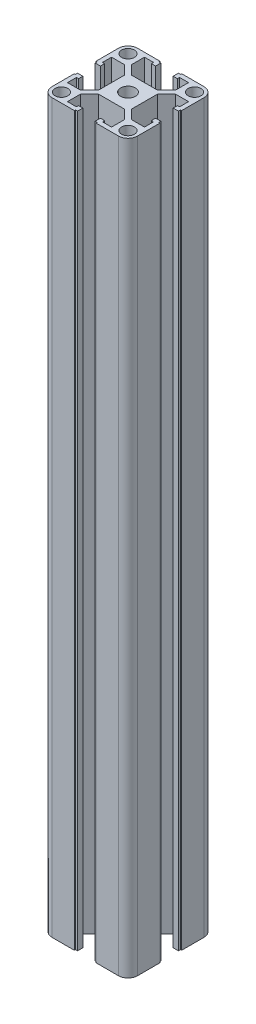
from build123d import *

# Parameters (mm, degrees)
SKETCH16_R             = 3.4
SKETCH16_R_2           = 3
MEMBER_1_DEPTH         = 340
HOLE_WIZARD_M8_3_D     = 6.9
HOLE_WIZARD_M8_3_DEPTH = 19.75
HOLE_WIZARD_M8_3_TIP   = 2.072969136


with BuildPart() as part:
    # Sketch16 → Member 1 (new body)
    with BuildSketch(Plane(origin=(0, 0, 0), x_dir=(-1, 0, 0), z_dir=(0, 1, 0))):
        with BuildLine():
            Line((-5.1, 20), (-5.1, 19.5))
            Line((-5.1, 19.5), (-4.1, 19.5))
            Line((-4.1, 19.5), (-4.1, 17))
            Line((-4.1, 17), (-6.1, 17))
            Line((-6.1, 17), (-6.1, 18))
            Line((-6.1, 18), (-10.3, 18))
            Line((-10.3, 18), (-10.3, 12))
            Line((-10.3, 12), (-6, 7.7))
            Line((-6, 7.7), (6, 7.7))
            Line((6, 7.7), (10.3, 12))
            Line((10.3, 12), (10.3, 18))
            Line((10.3, 18), (6.1, 18))
            Line((6.1, 18), (6.1, 17))
            Line((6.1, 17), (4.1, 17))
            Line((4.1, 17), (4.1, 19.5))
            Line((4.1, 19.5), (5.1, 19.5))
            Line((5.1, 19.5), (5.1, 20))
            Line((5.1, 20), (15.5, 20))
            ThreePointArc((15.5, 20), (18.681980515, 18.681980515), (20, 15.5))
            Line((20, 15.5), (20, 5.1))
            Line((20, 5.1), (19.5, 5.1))
            Line((19.5, 5.1), (19.5, 4.1))
            Line((19.5, 4.1), (17, 4.1))
            Line((17, 4.1), (17, 6.1))
            Line((17, 6.1), (18, 6.1))
            Line((18, 6.1), (18, 10.3))
            Line((18, 10.3), (12, 10.3))
            Line((12, 10.3), (7.7, 6))
            Line((7.7, 6), (7.7, -6))
            Line((7.7, -6), (12, -10.3))
            Line((12, -10.3), (18, -10.3))
            Line((18, -10.3), (18, -6.1))
            Line((18, -6.1), (17, -6.1))
            Line((17, -6.1), (17, -4.1))
            Line((17, -4.1), (19.5, -4.1))
            Line((19.5, -4.1), (19.5, -5.1))
            Line((19.5, -5.1), (20, -5.1))
            Line((20, -5.1), (20, -15.5))
            ThreePointArc((20, -15.5), (18.681980515, -18.681980515), (15.5, -20))
            Line((15.5, -20), (5.1, -20))
            Line((5.1, -20), (5.1, -19.5))
            Line((5.1, -19.5), (4.1, -19.5))
            Line((4.1, -19.5), (4.1, -17))
            Line((4.1, -17), (6.1, -17))
            Line((6.1, -17), (6.1, -18))
            Line((6.1, -18), (10.3, -18))
            Line((10.3, -18), (10.3, -12))
            Line((10.3, -12), (6, -7.7))
            Line((6, -7.7), (-6, -7.7))
            Line((-6, -7.7), (-10.3, -12))
            Line((-10.3, -12), (-10.3, -18))
            Line((-10.3, -18), (-6.1, -18))
            Line((-6.1, -18), (-6.1, -17))
            Line((-6.1, -17), (-4.1, -17))
            Line((-4.1, -17), (-4.1, -19.5))
            Line((-4.1, -19.5), (-5.1, -19.5))
            Line((-5.1, -19.5), (-5.1, -20))
            Line((-5.1, -20), (-15.5, -20))
            ThreePointArc((-15.5, -20), (-18.681980515, -18.681980515), (-20, -15.5))
            Line((-20, -15.5), (-20, -5.1))
            Line((-20, -5.1), (-19.5, -5.1))
            Line((-19.5, -5.1), (-19.5, -4.1))
            Line((-19.5, -4.1), (-17, -4.1))
            Line((-17, -4.1), (-17, -6.1))
            Line((-17, -6.1), (-18, -6.1))
            Line((-18, -6.1), (-18, -10.3))
            Line((-18, -10.3), (-12, -10.3))
            Line((-12, -10.3), (-7.7, -6))
            Line((-7.7, -6), (-7.7, 6))
            Line((-7.7, 6), (-12, 10.3))
            Line((-12, 10.3), (-18, 10.3))
            Line((-18, 10.3), (-18, 6.1))
            Line((-18, 6.1), (-17, 6.1))
            Line((-17, 6.1), (-17, 4.1))
            Line((-17, 4.1), (-19.5, 4.1))
            Line((-19.5, 4.1), (-19.5, 5.1))
            Line((-19.5, 5.1), (-20, 5.1))
            Line((-20, 5.1), (-20, 15.5))
            ThreePointArc((-20, 15.5), (-18.681980515, 18.681980515), (-15.5, 20))
            Line((-15.5, 20), (-5.1, 20))
        make_face()
        Circle(SKETCH16_R, mode=Mode.SUBTRACT)
        with Locations((-15.556349186, 15.556349186)):
            Circle(SKETCH16_R_2, mode=Mode.SUBTRACT)
        with Locations((15.556349186, 15.556349186)):
            Circle(SKETCH16_R_2, mode=Mode.SUBTRACT)
        with Locations((15.556349186, -15.556349186)):
            Circle(SKETCH16_R_2, mode=Mode.SUBTRACT)
        with Locations((-15.556349186, -15.556349186)):
            Circle(SKETCH16_R_2, mode=Mode.SUBTRACT)
    extrude(amount=MEMBER_1_DEPTH)

    # M8 螺纹孔3
    with Locations(Plane(origin=(0, 340, 0), x_dir=(1, 0, 0), z_dir=(0, 1, 0))):
        with Locations((0, 0)):
            Hole(HOLE_WIZARD_M8_3_D / 2, depth=HOLE_WIZARD_M8_3_DEPTH)
            with Locations((0, 0, -(HOLE_WIZARD_M8_3_DEPTH + HOLE_WIZARD_M8_3_TIP / 2))):  # 118° drill point
                Cone(0, HOLE_WIZARD_M8_3_D / 2, HOLE_WIZARD_M8_3_TIP, mode=Mode.SUBTRACT)


solid = part.part
